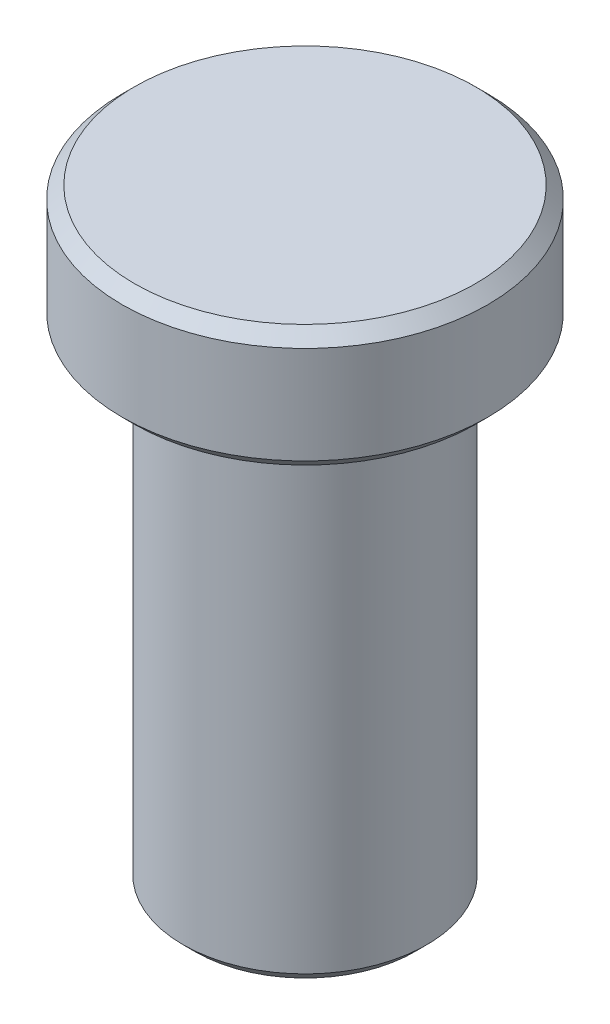
SolidWorks part; units mm, degrees
material "Q235-A"
ref_plane "Front Plane" through (0, 0, 0) normal (0, 0, 1) x (1, 0, 0)
ref_plane "Top Plane" through (0, 0, 0) normal (0, 1, 0) x (1, 0, 0)
ref_plane "Right Plane" through (0, 0, 0) normal (1, 0, 0) x (0, 0, -1)
sketch "Sketch2" plane through (0, 0, 0) normal (0, 1, 0) x (1, 0, 0)
  circle A0 centre (0, 0) radius 5
  dimension "D1" = 10
extrude "Boss-Extrude1" add sketch "Sketch2" along normal blind 20
sketch "Sketch3" plane through (0, 20, 0) normal (0, 1, 0) x (1, 0, 0)
  circle A0 centre (0, 0) radius 7.5
  dimension "D1" = 15
extrude "Boss-Extrude2" add sketch "Sketch3" along normal blind 5
chamfer "Chamfer2" distance 0.5 angle 45 3 edges at (0, 0, 5) (0, 25, 7.5) (0, 20, 7.5)
